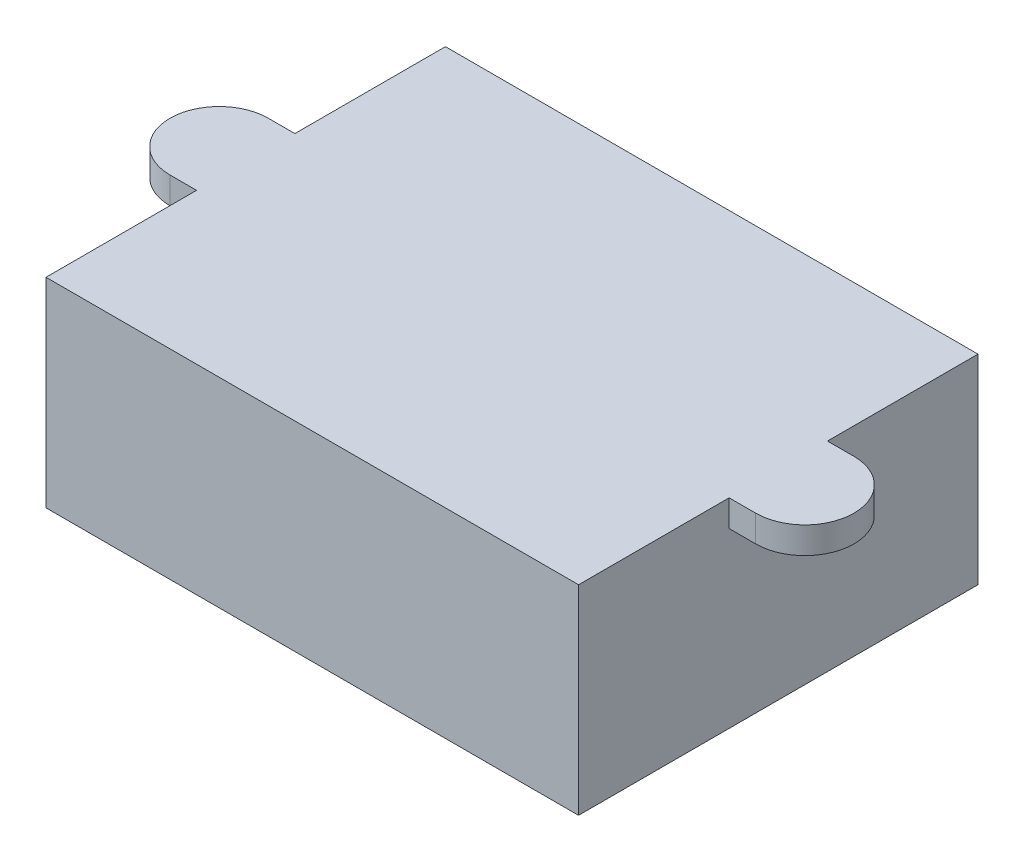
from build123d import *

# Parameters (mm, degrees)
SKETCH1_W           = 40
SKETCH1_H           = 30
BOSS_EXTRUDE1_DEPTH = 15
BOSS_EXTRUDE2_DEPTH = 2
SKETCH3_R           = 1.408779943
CUT_EXTRUDE1_DEPTH  = 5


with BuildPart() as part:
    # Sketch1 → Boss-Extrude1 (new body)
    with BuildSketch(Plane(origin=(0, 0, 0), x_dir=(1, 0, 0), z_dir=(0, 1, 0))):
        Rectangle(SKETCH1_W, SKETCH1_H)
    extrude(amount=BOSS_EXTRUDE1_DEPTH)

    # Sketch2 → Boss-Extrude2 (add)
    with BuildSketch(Plane(origin=(0, 15, 0), x_dir=(1, 0, 0), z_dir=(0, 1, 0))):
        with BuildLine():
            Line((-21.995796848, 3.691602268), (21.995796848, 3.691602268))
            ThreePointArc((21.995796848, 3.691602268), (25.687399116, 0), (21.995796848, -3.691602268))
            Line((21.995796848, -3.691602268), (-21.995796848, -3.691602268))
            ThreePointArc((-21.995796848, -3.691602268), (-25.687399116, 0), (-21.995796848, 3.691602268))
        make_face()
    extrude(amount=-BOSS_EXTRUDE2_DEPTH)

    # Sketch3 → Cut-Extrude1 (cut)
    with BuildSketch(Plane.XZ):
        with Locations(Location((-15.114073065, 6.951101682, 0), (0, 0, 270))):
            Circle(SKETCH3_R)
        with Locations(Location((-8.071509519, 6.951101682, 0), (0, 0, 270))):
            Circle(SKETCH3_R)
        with Locations(Location((-15.114073065, -6.448061429, 0), (0, 0, 270))):
            Circle(SKETCH3_R)
        with Locations(Location((-8.071509519, -6.448061429, 0), (0, 0, 270))):
            Circle(SKETCH3_R)
    extrude(amount=-CUT_EXTRUDE1_DEPTH, mode=Mode.SUBTRACT)


solid = part.part
